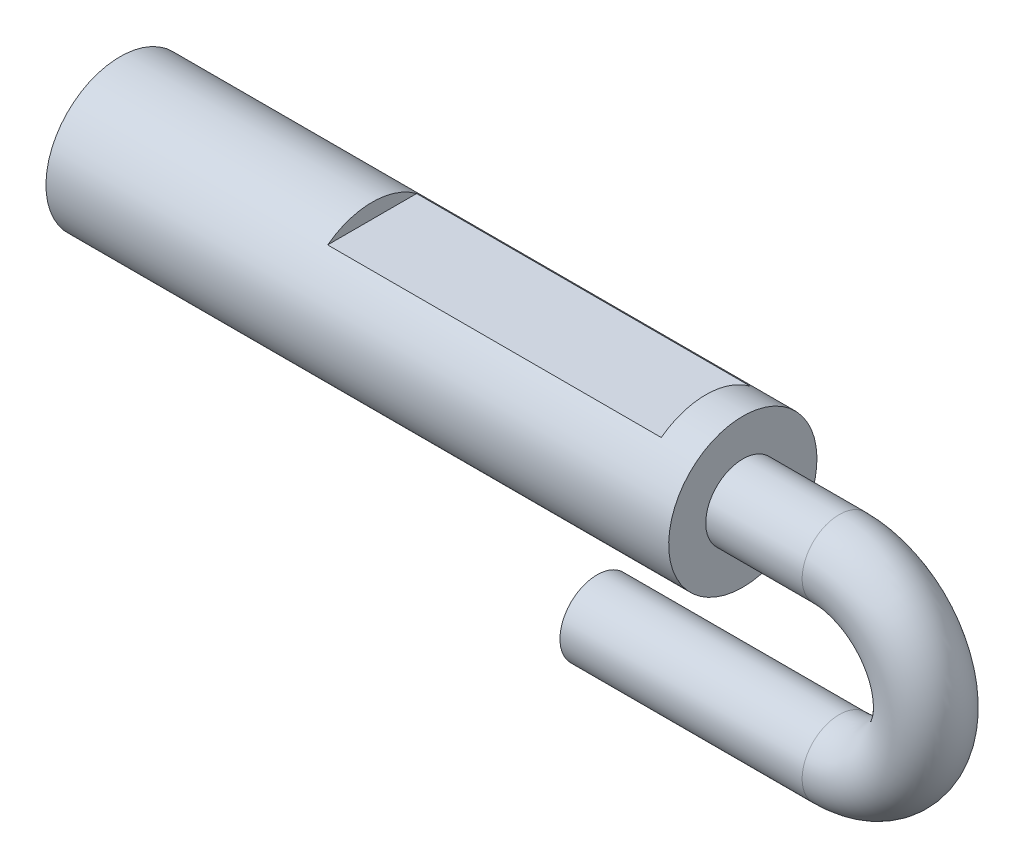
from build123d import *

# Parameters (mm, degrees)
SKETCH_1_W          = 84
SKETCH_1_H          = 10
SKETCH_2_W          = 45
SKETCH_2_H          = 40.446231626
CUT_EXTRUDE_1_DEPTH = 2
SWEEP_1_PROFILE_R   = 5


with BuildPart() as part:
    # 草图1 → 旋转1 (revolve)
    with BuildSketch(Plane.XY, mode=Mode.PRIVATE) as revolve_1_sk:
        with Locations((0, 5)):
            Rectangle(SKETCH_1_W, SKETCH_1_H)
    revolve(revolve_1_sk.sketch.rotate(Axis((-42, 0, 0), (1, 0, 0)), 180), axis=Axis((-42, 0, 0), (1, 0, 0)))

    # 草图2 → 切除-拉伸1 (cut)
    with BuildSketch(Plane(origin=(0, 10, 0), x_dir=(1, 0, 0), z_dir=(0, 1, 0))):
        with Locations((14.5, -3.02134906)):
            Rectangle(SKETCH_2_W, SKETCH_2_H)
    extrude(amount=-CUT_EXTRUDE_1_DEPTH, mode=Mode.SUBTRACT)

    # 扫描1: sweep along a path in 草图3
    with BuildLine(Plane.XY) as sweep_1_path:
        Line((42, 0), (55.00002565, 0))
        ThreePointArc((55.00002565, 0), (66.683449814, -11.683424164), (55.00002565, -23.366848328))
        Line((55.00002565, -23.366848328), (22.334289366, -23.366848328))
    # 扫描1 profile (on start of the path) → 扫描1 (sweep)
    with BuildSketch(Plane.YZ.offset(42)):
        Circle(SWEEP_1_PROFILE_R)
    sweep(path=sweep_1_path.line)


solid = part.part
